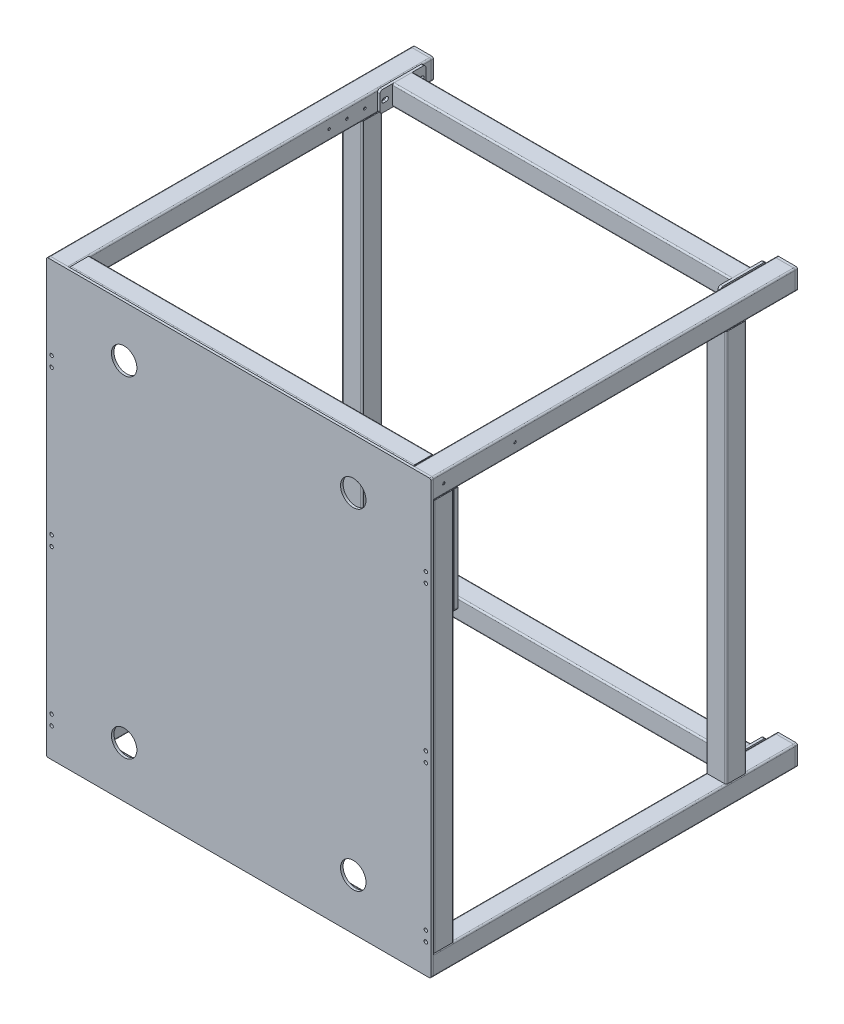
from build123d import *

# Parameters (mm, degrees)
SKETCH_1_W             = 755
SKETCH_1_H             = 850
EXTRUDE_1_DEPTH        = 5
EXTRUDE_3_DEPTH        = 710
EXTRUDE_3_2_DEPTH      = 710
EXTRUDE_3_3_DEPTH      = 710
EXTRUDE_3_4_DEPTH      = 710
FILLET_1_R             = 3
EXTRUDE_4_DEPTH        = 675
EXTRUDE_4_2_DEPTH      = 675
EXTRUDE_5_DEPTH        = 770
EXTRUDE_5_2_DEPTH      = 770
SKETCH_6_R             = 3.4
CUT_EXTRUDE_1_DEPTH    = 30
SKETCH_7_R             = 9.5
EXTRUDE_6_DEPTH        = 5
EXTRUDE_6_2_DEPTH      = 5
EXTRUDE_6_3_DEPTH      = 5
EXTRUDE_6_4_DEPTH      = 5
SKETCH_8_W             = 60
SKETCH_8_H             = 210
EXTRUDE_7_DEPTH        = 8
SKETCH_9_R             = 3.4
CUT_EXTRUDE_2_DEPTH    = 10
FILLET_2_R             = 5
EXTRUDE_8_DEPTH        = 770
EXTRUDE_8_2_DEPTH      = 770
SKETCH_11_W            = 90
SKETCH_11_H            = 40
EXTRUDE_9_DEPTH        = 5
FILLET_3_R             = 5
CUT_EXTRUDE_3_DEPTH    = 5
EXTRUDE_10_DEPTH       = 664
EXTRUDE_11_DEPTH       = 5
CUT_EXTRUDE_START      = -2
SKETCH_15_R            = 2.5
CUT_EXTRUDE_4_DEPTH    = 679
PATTERN_LINEAR_1_COUNT = 2
PATTERN_LINEAR_1_PITCH = 810
SKETCH_16_R            = 25
CUT_EXTRUDE_5_DEPTH    = 10
SKETCH_17_R            = 2.5
CUT_EXTRUDE_6_DEPTH    = 1.5


with BuildPart() as part:
    # 草图1 → 凸台-拉伸1 (new body)
    with BuildSketch(Plane.XY):
        Rectangle(SKETCH_1_W, SKETCH_1_H)
    extrude(amount=EXTRUDE_1_DEPTH)

    # 圆角1
    fillet_1_edges = [part.edges().sort_by_distance(p)[0] for p in [
        (377.5, -425, 2.5),
        (-377.5, -425, 2.5),
        (-377.5, 425, 2.5),
        (377.5, 425, 2.5),
    ]]
    fillet(fillet_1_edges, radius=FILLET_1_R)


with BuildPart() as body_2:
    # 草图3 → 凸台-拉伸3 (new body)
    with BuildSketch(Plane(origin=(0, 0, 0), x_dir=(-1, 0, 0), z_dir=(0, 0, -1))):
        with BuildLine():
            Line((374.5, 385), (340.5, 385))
            ThreePointArc((340.5, 385), (338.378679656, 385.878679656), (337.5, 388))
            Line((337.5, 388), (337.5, 422))
            ThreePointArc((337.5, 422), (338.378679656, 424.121320344), (340.5, 425))
            Line((340.5, 425), (374.5, 425))
            ThreePointArc((374.5, 425), (376.621320344, 424.121320344), (377.5, 422))
            Line((377.5, 422), (377.5, 388))
            ThreePointArc((377.5, 388), (376.621320344, 385.878679656), (374.5, 385))
        make_face()
        with BuildLine():
            Line((339.5, 388), (339.5, 422))
            ThreePointArc((339.5, 422), (339.792893219, 422.707106781), (340.5, 423))
            Line((340.5, 423), (374.5, 423))
            ThreePointArc((374.5, 423), (375.207106781, 422.707106781), (375.5, 422))
            Line((375.5, 422), (375.5, 388))
            ThreePointArc((375.5, 388), (375.207106781, 387.292893219), (374.5, 387))
            Line((374.5, 387), (340.5, 387))
            ThreePointArc((340.5, 387), (339.792893219, 387.292893219), (339.5, 388))
        make_face(mode=Mode.SUBTRACT)
    extrude(amount=EXTRUDE_3_DEPTH)


with BuildPart() as body_3:
    # 草图3 → Extrude 3 2 (new body)
    with BuildSketch(Plane(origin=(0, 0, 0), x_dir=(-1, 0, 0), z_dir=(0, 0, -1))):
        with BuildLine():
            Line((374.5, -425), (340.5, -425))
            ThreePointArc((340.5, -425), (338.378679656, -424.121320344), (337.5, -422))
            Line((337.5, -422), (337.5, -388))
            ThreePointArc((337.5, -388), (338.378679656, -385.878679656), (340.5, -385))
            Line((340.5, -385), (374.5, -385))
            ThreePointArc((374.5, -385), (376.621320344, -385.878679656), (377.5, -388))
            Line((377.5, -388), (377.5, -422))
            ThreePointArc((377.5, -422), (376.621320344, -424.121320344), (374.5, -425))
        make_face()
        with BuildLine():
            Line((339.5, -422), (339.5, -388))
            ThreePointArc((339.5, -388), (339.792893219, -387.292893219), (340.5, -387))
            Line((340.5, -387), (374.5, -387))
            ThreePointArc((374.5, -387), (375.207106781, -387.292893219), (375.5, -388))
            Line((375.5, -388), (375.5, -422))
            ThreePointArc((375.5, -422), (375.207106781, -422.707106781), (374.5, -423))
            Line((374.5, -423), (340.5, -423))
            ThreePointArc((340.5, -423), (339.792893219, -422.707106781), (339.5, -422))
        make_face(mode=Mode.SUBTRACT)
    extrude(amount=EXTRUDE_3_2_DEPTH)


with BuildPart() as body_4:
    # 草图3 → Extrude 3 3 (new body)
    with BuildSketch(Plane(origin=(0, 0, 0), x_dir=(-1, 0, 0), z_dir=(0, 0, -1))):
        with BuildLine():
            Line((-340.5, -425), (-374.5, -425))
            ThreePointArc((-374.5, -425), (-376.621320344, -424.121320344), (-377.5, -422))
            Line((-377.5, -422), (-377.5, -388))
            ThreePointArc((-377.5, -388), (-376.621320344, -385.878679656), (-374.5, -385))
            Line((-374.5, -385), (-340.5, -385))
            ThreePointArc((-340.5, -385), (-338.378679656, -385.878679656), (-337.5, -388))
            Line((-337.5, -388), (-337.5, -422))
            ThreePointArc((-337.5, -422), (-338.378679656, -424.121320344), (-340.5, -425))
        make_face()
        with BuildLine():
            Line((-375.5, -422), (-375.5, -388))
            ThreePointArc((-375.5, -388), (-375.207106781, -387.292893219), (-374.5, -387))
            Line((-374.5, -387), (-340.5, -387))
            ThreePointArc((-340.5, -387), (-339.792893219, -387.292893219), (-339.5, -388))
            Line((-339.5, -388), (-339.5, -422))
            ThreePointArc((-339.5, -422), (-339.792893219, -422.707106781), (-340.5, -423))
            Line((-340.5, -423), (-374.5, -423))
            ThreePointArc((-374.5, -423), (-375.207106781, -422.707106781), (-375.5, -422))
        make_face(mode=Mode.SUBTRACT)
    extrude(amount=EXTRUDE_3_3_DEPTH)


with BuildPart() as body_5:
    # 草图3 → Extrude 3 4 (new body)
    with BuildSketch(Plane(origin=(0, 0, 0), x_dir=(-1, 0, 0), z_dir=(0, 0, -1))):
        with BuildLine():
            Line((-340.5, 385), (-374.5, 385))
            ThreePointArc((-374.5, 385), (-376.621320344, 385.878679656), (-377.5, 388))
            Line((-377.5, 388), (-377.5, 422))
            ThreePointArc((-377.5, 422), (-376.621320344, 424.121320344), (-374.5, 425))
            Line((-374.5, 425), (-340.5, 425))
            ThreePointArc((-340.5, 425), (-338.378679656, 424.121320344), (-337.5, 422))
            Line((-337.5, 422), (-337.5, 388))
            ThreePointArc((-337.5, 388), (-338.378679656, 385.878679656), (-340.5, 385))
        make_face()
        with BuildLine():
            Line((-375.5, 388), (-375.5, 422))
            ThreePointArc((-375.5, 422), (-375.207106781, 422.707106781), (-374.5, 423))
            Line((-374.5, 423), (-340.5, 423))
            ThreePointArc((-340.5, 423), (-339.792893219, 422.707106781), (-339.5, 422))
            Line((-339.5, 422), (-339.5, 388))
            ThreePointArc((-339.5, 388), (-339.792893219, 387.292893219), (-340.5, 387))
            Line((-340.5, 387), (-374.5, 387))
            ThreePointArc((-374.5, 387), (-375.207106781, 387.292893219), (-375.5, 388))
        make_face(mode=Mode.SUBTRACT)
    extrude(amount=EXTRUDE_3_4_DEPTH)


with BuildPart() as body_6:
    # 草图4 → 凸台-拉伸4 (new body)
    with BuildSketch(Plane(origin=(-337.5, 0, 0), x_dir=(0, 0, -1), z_dir=(1, 0, 0))):
        with BuildLine():
            Line((37, 385), (3, 385))
            ThreePointArc((3, 385), (0.878679656, 385.878679656), (0, 388))
            Line((0, 388), (0, 422))
            ThreePointArc((0, 422), (0.878679656, 424.121320344), (3, 425))
            Line((3, 425), (37, 425))
            ThreePointArc((37, 425), (39.121320344, 424.121320344), (40, 422))
            Line((40, 422), (40, 388))
            ThreePointArc((40, 388), (39.121320344, 385.878679656), (37, 385))
        make_face()
        with BuildLine():
            Line((2, 388), (2, 422))
            ThreePointArc((2, 422), (2.292893219, 422.707106781), (3, 423))
            Line((3, 423), (37, 423))
            ThreePointArc((37, 423), (37.707106781, 422.707106781), (38, 422))
            Line((38, 422), (38, 388))
            ThreePointArc((38, 388), (37.707106781, 387.292893219), (37, 387))
            Line((37, 387), (3, 387))
            ThreePointArc((3, 387), (2.292893219, 387.292893219), (2, 388))
        make_face(mode=Mode.SUBTRACT)
    extrude(amount=EXTRUDE_4_DEPTH)


with BuildPart() as body_7:
    # 草图4 → Extrude 4 2 (new body)
    with BuildSketch(Plane(origin=(-337.5, 0, 0), x_dir=(0, 0, -1), z_dir=(1, 0, 0))):
        with BuildLine():
            Line((37, -425), (3, -425))
            ThreePointArc((3, -425), (0.878679656, -424.121320344), (0, -422))
            Line((0, -422), (0, -388))
            ThreePointArc((0, -388), (0.878679656, -385.878679656), (3, -385))
            Line((3, -385), (37, -385))
            ThreePointArc((37, -385), (39.121320344, -385.878679656), (40, -388))
            Line((40, -388), (40, -422))
            ThreePointArc((40, -422), (39.121320344, -424.121320344), (37, -425))
        make_face()
        with BuildLine():
            Line((2, -422), (2, -388))
            ThreePointArc((2, -388), (2.292893219, -387.292893219), (3, -387))
            Line((3, -387), (37, -387))
            ThreePointArc((37, -387), (37.707106781, -387.292893219), (38, -388))
            Line((38, -388), (38, -422))
            ThreePointArc((38, -422), (37.707106781, -422.707106781), (37, -423))
            Line((37, -423), (3, -423))
            ThreePointArc((3, -423), (2.292893219, -422.707106781), (2, -422))
        make_face(mode=Mode.SUBTRACT)
    extrude(amount=EXTRUDE_4_2_DEPTH)


with BuildPart() as body_8:
    # 草图5 → 凸台-拉伸5 (new body)
    with BuildSketch(Plane(origin=(0, -385, 0), x_dir=(1, 0, 0), z_dir=(0, 1, 0))):
        with BuildLine():
            Line((374.5, 0), (340.5, 0))
            ThreePointArc((340.5, 0), (338.378679656, 0.878679656), (337.5, 3))
            Line((337.5, 3), (337.5, 37))
            ThreePointArc((337.5, 37), (338.378679656, 39.121320344), (340.5, 40))
            Line((340.5, 40), (374.5, 40))
            ThreePointArc((374.5, 40), (376.621320344, 39.121320344), (377.5, 37))
            Line((377.5, 37), (377.5, 3))
            ThreePointArc((377.5, 3), (376.621320344, 0.878679656), (374.5, 0))
        make_face()
        with BuildLine():
            Line((339.5, 3), (339.5, 37))
            ThreePointArc((339.5, 37), (339.792893219, 37.707106781), (340.5, 38))
            Line((340.5, 38), (374.5, 38))
            ThreePointArc((374.5, 38), (375.207106781, 37.707106781), (375.5, 37))
            Line((375.5, 37), (375.5, 3))
            ThreePointArc((375.5, 3), (375.207106781, 2.292893219), (374.5, 2))
            Line((374.5, 2), (340.5, 2))
            ThreePointArc((340.5, 2), (339.792893219, 2.292893219), (339.5, 3))
        make_face(mode=Mode.SUBTRACT)
    extrude(amount=EXTRUDE_5_DEPTH)


with BuildPart() as body_9:
    # 草图5 → Extrude 5 2 (new body)
    with BuildSketch(Plane(origin=(0, -385, 0), x_dir=(1, 0, 0), z_dir=(0, 1, 0))):
        with BuildLine():
            Line((-340.5, 0), (-374.5, 0))
            ThreePointArc((-374.5, 0), (-376.621320344, 0.878679656), (-377.5, 3))
            Line((-377.5, 3), (-377.5, 37))
            ThreePointArc((-377.5, 37), (-376.621320344, 39.121320344), (-374.5, 40))
            Line((-374.5, 40), (-340.5, 40))
            ThreePointArc((-340.5, 40), (-338.378679656, 39.121320344), (-337.5, 37))
            Line((-337.5, 37), (-337.5, 3))
            ThreePointArc((-337.5, 3), (-338.378679656, 0.878679656), (-340.5, 0))
        make_face()
        with BuildLine():
            Line((-375.5, 3), (-375.5, 37))
            ThreePointArc((-375.5, 37), (-375.207106781, 37.707106781), (-374.5, 38))
            Line((-374.5, 38), (-340.5, 38))
            ThreePointArc((-340.5, 38), (-339.792893219, 37.707106781), (-339.5, 37))
            Line((-339.5, 37), (-339.5, 3))
            ThreePointArc((-339.5, 3), (-339.792893219, 2.292893219), (-340.5, 2))
            Line((-340.5, 2), (-374.5, 2))
            ThreePointArc((-374.5, 2), (-375.207106781, 2.292893219), (-375.5, 3))
        make_face(mode=Mode.SUBTRACT)
    extrude(amount=EXTRUDE_5_2_DEPTH)


with BuildPart() as cut_extrude_1_tool:
    # 草图6 → 切除-拉伸1 (new body)
    with BuildSketch(Plane.XY.offset(5)):
        with Locations(Location((-367.5, -367.5, 0), (0, 0, 180))):
            Circle(SKETCH_6_R)
        with Locations(Location((-367.5, -347.5, 0), (0, 0, 180))):
            Circle(SKETCH_6_R)
        with Locations(Location((367.5, 262.5, 0), (0, 0, 180))):
            Circle(SKETCH_6_R)
        with Locations(Location((-367.5, -62.5, 0), (0, 0, 180))):
            Circle(SKETCH_6_R)
        with Locations(Location((-367.5, -42.5, 0), (0, 0, 180))):
            Circle(SKETCH_6_R)
        with Locations(Location((-367.5, 242.5, 0), (0, 0, 180))):
            Circle(SKETCH_6_R)
        with Locations(Location((-367.5, 262.5, 0), (0, 0, 180))):
            Circle(SKETCH_6_R)
        with Locations(Location((367.5, 242.5, 0), (0, 0, 180))):
            Circle(SKETCH_6_R)
        with Locations(Location((367.5, -42.5, 0), (0, 0, 180))):
            Circle(SKETCH_6_R)
        with Locations(Location((367.5, -62.5, 0), (0, 0, 180))):
            Circle(SKETCH_6_R)
        with Locations(Location((367.5, -347.5, 0), (0, 0, 180))):
            Circle(SKETCH_6_R)
        with Locations(Location((367.5, -367.5, 0), (0, 0, 180))):
            Circle(SKETCH_6_R)
    extrude(amount=-CUT_EXTRUDE_1_DEPTH)


with BuildPart() as part_1:
    add(part.part)

    # 切除-拉伸1: cut by cut_extrude_1_tool
    add(cut_extrude_1_tool.part, mode=Mode.SUBTRACT)

    # 草图16 → 切除-拉伸5 (cut)
    with BuildSketch(Plane.XY.offset(5)):
        with Locations((-225, 325)):
            Circle(SKETCH_16_R)
        with Locations((225, 325)):
            Circle(SKETCH_16_R)
        with Locations((225, -325)):
            Circle(SKETCH_16_R)
        with Locations((-225, -325)):
            Circle(SKETCH_16_R)
    extrude(amount=-CUT_EXTRUDE_5_DEPTH, mode=Mode.SUBTRACT)


with BuildPart() as body_8_1:
    add(body_8.part)

    # 切除-拉伸1: cut by cut_extrude_1_tool
    add(cut_extrude_1_tool.part, mode=Mode.SUBTRACT)


with BuildPart() as body_9_1:
    add(body_9.part)

    # 切除-拉伸1: cut by cut_extrude_1_tool
    add(cut_extrude_1_tool.part, mode=Mode.SUBTRACT)


with BuildPart() as body_10:
    # 草图7 → 凸台-拉伸6 (new body)
    with BuildSketch(Plane(origin=(0, 0, -710), x_dir=(-1, 0, 0), z_dir=(0, 0, -1))):
        with BuildLine():
            Line((337.5, 422), (337.5, 388))
            ThreePointArc((337.5, 388), (338.378679656, 385.878679656), (340.5, 385))
            Line((340.5, 385), (374.5, 385))
            ThreePointArc((374.5, 385), (376.621320344, 385.878679656), (377.5, 388))
            Line((377.5, 388), (377.5, 422))
            ThreePointArc((377.5, 422), (376.621320344, 424.121320344), (374.5, 425))
            Line((374.5, 425), (340.5, 425))
            ThreePointArc((340.5, 425), (338.378679656, 424.121320344), (337.5, 422))
        make_face()
        with Locations((357.5, 405)):
            Circle(SKETCH_7_R, mode=Mode.SUBTRACT)
    extrude(amount=EXTRUDE_6_DEPTH)


with BuildPart() as body_11:
    # 草图7 → Extrude 6 2 (new body)
    with BuildSketch(Plane(origin=(0, 0, -710), x_dir=(-1, 0, 0), z_dir=(0, 0, -1))):
        with BuildLine():
            Line((337.5, -388), (337.5, -422))
            ThreePointArc((337.5, -422), (338.378679656, -424.121320344), (340.5, -425))
            Line((340.5, -425), (374.5, -425))
            ThreePointArc((374.5, -425), (376.621320344, -424.121320344), (377.5, -422))
            Line((377.5, -422), (377.5, -388))
            ThreePointArc((377.5, -388), (376.621320344, -385.878679656), (374.5, -385))
            Line((374.5, -385), (340.5, -385))
            ThreePointArc((340.5, -385), (338.378679656, -385.878679656), (337.5, -388))
        make_face()
        with Locations((357.5, -405)):
            Circle(SKETCH_7_R, mode=Mode.SUBTRACT)
    extrude(amount=EXTRUDE_6_2_DEPTH)


with BuildPart() as body_12:
    # 草图7 → Extrude 6 3 (new body)
    with BuildSketch(Plane(origin=(0, 0, -710), x_dir=(-1, 0, 0), z_dir=(0, 0, -1))):
        with BuildLine():
            Line((-377.432040581, -388), (-377.432040581, -422))
            ThreePointArc((-377.432040581, -422), (-376.553360924, -424.121320344), (-374.432040581, -425))
            Line((-374.432040581, -425), (-340.432040581, -425))
            ThreePointArc((-340.432040581, -425), (-338.310720237, -424.121320344), (-337.432040581, -422))
            Line((-337.432040581, -422), (-337.432040581, -388))
            ThreePointArc((-337.432040581, -388), (-338.310720237, -385.878679656), (-340.432040581, -385))
            Line((-340.432040581, -385), (-374.432040581, -385))
            ThreePointArc((-374.432040581, -385), (-376.553360924, -385.878679656), (-377.432040581, -388))
        make_face()
        with Locations((-357.432040581, -405)):
            Circle(SKETCH_7_R, mode=Mode.SUBTRACT)
    extrude(amount=EXTRUDE_6_3_DEPTH)


with BuildPart() as body_13:
    # 草图7 → Extrude 6 4 (new body)
    with BuildSketch(Plane(origin=(0, 0, -710), x_dir=(-1, 0, 0), z_dir=(0, 0, -1))):
        with BuildLine():
            Line((-377.5, 422), (-377.5, 388))
            ThreePointArc((-377.5, 388), (-376.621320344, 385.878679656), (-374.5, 385))
            Line((-374.5, 385), (-340.5, 385))
            ThreePointArc((-340.5, 385), (-338.378679656, 385.878679656), (-337.5, 388))
            Line((-337.5, 388), (-337.5, 422))
            ThreePointArc((-337.5, 422), (-338.378679656, 424.121320344), (-340.5, 425))
            Line((-340.5, 425), (-374.5, 425))
            ThreePointArc((-374.5, 425), (-376.621320344, 424.121320344), (-377.5, 422))
        make_face()
        with Locations((-357.5, 405)):
            Circle(SKETCH_7_R, mode=Mode.SUBTRACT)
    extrude(amount=EXTRUDE_6_4_DEPTH)


with BuildPart() as body_14:
    # 草图8 → 凸台-拉伸7 (new body)
    with BuildSketch(Plane(origin=(0, 0, -40), x_dir=(-1, 0, 0), z_dir=(0, 0, -1))):
        with Locations((-347.5, 280)):
            Rectangle(SKETCH_8_W, SKETCH_8_H)
    extrude(amount=EXTRUDE_7_DEPTH)


with BuildPart() as cut_extrude_2_tool:
    # 草图9 → 切除-拉伸2 (new body)
    with BuildSketch(Plane(origin=(0, 0, -48), x_dir=(-1, 0, 0), z_dir=(0, 0, -1))):
        with Locations((-366.5, 187.5)):
            Circle(SKETCH_9_R)
        with Locations((-328.5, 187.5)):
            Circle(SKETCH_9_R)
        with Locations((-366.5, 352.5)):
            Circle(SKETCH_9_R)
        with Locations((-328.5, 352.5)):
            Circle(SKETCH_9_R)
    extrude(amount=-CUT_EXTRUDE_2_DEPTH)


with BuildPart() as body_8_2:
    add(body_8_1.part)

    # 切除-拉伸2: cut by cut_extrude_2_tool
    add(cut_extrude_2_tool.part, mode=Mode.SUBTRACT)


with BuildPart() as body_14_1:
    add(body_14.part)

    # 切除-拉伸2: cut by cut_extrude_2_tool
    add(cut_extrude_2_tool.part, mode=Mode.SUBTRACT)

    # 圆角2
    fillet_2_edges = [body_14_1.edges().sort_by_distance(p)[0] for p in [
        (317.5, 385, -44),
        (317.5, 175, -44),
        (377.5, 175, -44),
    ]]
    fillet(fillet_2_edges, radius=FILLET_2_R)


with BuildPart() as body_15:
    # 草图10 → 凸台-拉伸8 (new body)
    with BuildSketch(Plane.XZ.offset(-385)):
        with BuildLine():
            Line((-340.5, -615), (-374.5, -615))
            ThreePointArc((-374.5, -615), (-376.621320344, -614.121320344), (-377.5, -612))
            Line((-377.5, -612), (-377.5, -578))
            ThreePointArc((-377.5, -578), (-376.621320344, -575.878679656), (-374.5, -575))
            Line((-374.5, -575), (-340.5, -575))
            ThreePointArc((-340.5, -575), (-338.378679656, -575.878679656), (-337.5, -578))
            Line((-337.5, -578), (-337.5, -612))
            ThreePointArc((-337.5, -612), (-338.378679656, -614.121320344), (-340.5, -615))
        make_face()
        with BuildLine():
            Line((-375.5, -612), (-375.5, -578))
            ThreePointArc((-375.5, -578), (-375.207106781, -577.292893219), (-374.5, -577))
            Line((-374.5, -577), (-340.5, -577))
            ThreePointArc((-340.5, -577), (-339.792893219, -577.292893219), (-339.5, -578))
            Line((-339.5, -578), (-339.5, -612))
            ThreePointArc((-339.5, -612), (-339.792893219, -612.707106781), (-340.5, -613))
            Line((-340.5, -613), (-374.5, -613))
            ThreePointArc((-374.5, -613), (-375.207106781, -612.707106781), (-375.5, -612))
        make_face(mode=Mode.SUBTRACT)
    extrude(amount=EXTRUDE_8_DEPTH)


with BuildPart() as body_16:
    # 草图10 → Extrude 8 2 (new body)
    with BuildSketch(Plane.XZ.offset(-385)):
        with BuildLine():
            Line((374.5, -615), (340.5, -615))
            ThreePointArc((340.5, -615), (338.378679656, -614.121320344), (337.5, -612))
            Line((337.5, -612), (337.5, -578))
            ThreePointArc((337.5, -578), (338.378679656, -575.878679656), (340.5, -575))
            Line((340.5, -575), (374.5, -575))
            ThreePointArc((374.5, -575), (376.621320344, -575.878679656), (377.5, -578))
            Line((377.5, -578), (377.5, -612))
            ThreePointArc((377.5, -612), (376.621320344, -614.121320344), (374.5, -615))
        make_face()
        with BuildLine():
            Line((339.5, -612), (339.5, -578))
            ThreePointArc((339.5, -578), (339.792893219, -577.292893219), (340.5, -577))
            Line((340.5, -577), (374.5, -577))
            ThreePointArc((374.5, -577), (375.207106781, -577.292893219), (375.5, -578))
            Line((375.5, -578), (375.5, -612))
            ThreePointArc((375.5, -612), (375.207106781, -612.707106781), (374.5, -613))
            Line((374.5, -613), (340.5, -613))
            ThreePointArc((340.5, -613), (339.792893219, -612.707106781), (339.5, -612))
        make_face(mode=Mode.SUBTRACT)
    extrude(amount=EXTRUDE_8_2_DEPTH)


with BuildPart() as body_17:
    # 草图11 → 凸台-拉伸9 (new body)
    with BuildSketch(Plane(origin=(-337.5, 0, 0), x_dir=(0, 0, -1), z_dir=(1, 0, 0))):
        with Locations((650, -405)):
            Rectangle(SKETCH_11_W, SKETCH_11_H)
    extrude(amount=EXTRUDE_9_DEPTH)

    # 圆角3
    fillet_3_edges = [body_17.edges().sort_by_distance(p)[0] for p in [
        (-335, -385, -605),
        (-335, -385, -695),
        (-335, -425, -695),
        (-335, -425, -605),
    ]]
    fillet(fillet_3_edges, radius=FILLET_3_R)

    # 草图12 → 切除-拉伸3 (cut)
    with BuildSketch(Plane(origin=(-332.5, 0, 0), x_dir=(0, 0, -1), z_dir=(1, 0, 0))):
        with BuildLine():
            Line((612.5, -401), (617.5, -401))
            ThreePointArc((617.5, -401), (621.5, -405), (617.5, -409))
            Line((617.5, -409), (612.5, -409))
            ThreePointArc((612.5, -409), (608.5, -405), (612.5, -401))
        make_face()
        with BuildLine():
            Line((687.5, -401), (682.5, -401))
            ThreePointArc((682.5, -401), (678.5, -405), (682.5, -409))
            Line((682.5, -409), (687.5, -409))
            ThreePointArc((687.5, -409), (691.5, -405), (687.5, -401))
        make_face()
    extrude(amount=-CUT_EXTRUDE_3_DEPTH, mode=Mode.SUBTRACT)


with BuildPart() as body_18:
    # 草图13 → 凸台-拉伸10 (new body)
    with BuildSketch(Plane(origin=(-332.5, 0, 0), x_dir=(0, 0, -1), z_dir=(1, 0, 0))):
        with BuildLine():
            Line((667, -425), (633, -425))
            ThreePointArc((633, -425), (630.878679656, -424.121320344), (630, -422))
            Line((630, -422), (630, -388))
            ThreePointArc((630, -388), (630.878679656, -385.878679656), (633, -385))
            Line((633, -385), (667, -385))
            ThreePointArc((667, -385), (669.121320344, -385.878679656), (670, -388))
            Line((670, -388), (670, -422))
            ThreePointArc((670, -422), (669.121320344, -424.121320344), (667, -425))
        make_face()
        with BuildLine():
            Line((632, -422), (632, -388))
            ThreePointArc((632, -388), (632.292893219, -387.292893219), (633, -387))
            Line((633, -387), (667, -387))
            ThreePointArc((667, -387), (667.707106781, -387.292893219), (668, -388))
            Line((668, -388), (668, -422))
            ThreePointArc((668, -422), (667.707106781, -422.707106781), (667, -423))
            Line((667, -423), (633, -423))
            ThreePointArc((633, -423), (632.292893219, -422.707106781), (632, -422))
        make_face(mode=Mode.SUBTRACT)
    extrude(amount=EXTRUDE_10_DEPTH)


with BuildPart() as body_19:
    # 草图14 → 凸台-拉伸11 (new body)
    with BuildSketch(Plane(origin=(331.5, 0, 0), x_dir=(0, 0, -1), z_dir=(1, 0, 0))):
        with BuildLine():
            Line((610, -425), (690, -425))
            ThreePointArc((690, -425), (693.535533906, -423.535533906), (695, -420))
            Line((695, -420), (695, -390))
            ThreePointArc((695, -390), (693.535533906, -386.464466094), (690, -385))
            Line((690, -385), (610, -385))
            ThreePointArc((610, -385), (606.464466094, -386.464466094), (605, -390))
            Line((605, -390), (605, -420))
            ThreePointArc((605, -420), (606.464466094, -423.535533906), (610, -425))
        make_face()
        with BuildLine():
            Line((687.5, -401), (682.5, -401))
            ThreePointArc((682.5, -401), (678.5, -405), (682.5, -409))
            Line((682.5, -409), (687.5, -409))
            ThreePointArc((687.5, -409), (691.5, -405), (687.5, -401))
        make_face(mode=Mode.SUBTRACT)
        with BuildLine():
            Line((612.5, -409), (617.5, -409))
            ThreePointArc((617.5, -409), (621.5, -405), (617.5, -401))
            Line((617.5, -401), (612.5, -401))
            ThreePointArc((612.5, -401), (608.5, -405), (612.5, -409))
        make_face(mode=Mode.SUBTRACT)
    extrude(amount=EXTRUDE_11_DEPTH)


with BuildPart() as cut_extrude_4_tool:
    # 草图15 → 切除-拉伸4 (new body)
    with BuildSketch(Plane(origin=(-337.5, 0, 0), x_dir=(0, 0, -1), z_dir=(1, 0, 0)).offset(CUT_EXTRUDE_START)):
        with Locations((685, -405)):
            Circle(SKETCH_15_R)
        with Locations((650, -405)):
            Circle(SKETCH_15_R)
        with Locations((615, -405)):
            Circle(SKETCH_15_R)
        with Locations((580, -405)):
            Circle(SKETCH_15_R)
        with Locations((545, -405)):
            Circle(SKETCH_15_R)
        with Locations((510, -405)):
            Circle(SKETCH_15_R)
        with Locations((510, 405)):
            Circle(SKETCH_15_R)
        with Locations((545, 405)):
            Circle(SKETCH_15_R)
        with Locations((580, 405)):
            Circle(SKETCH_15_R)
        with Locations((615, 405)):
            Circle(SKETCH_15_R)
        with Locations((650, 405)):
            Circle(SKETCH_15_R)
        with Locations((685, 405)):
            Circle(SKETCH_15_R)
    extrude(amount=CUT_EXTRUDE_4_DEPTH)


with BuildPart() as body_2_1:
    add(body_2.part)

    # 切除-拉伸4: cut by cut_extrude_4_tool
    add(cut_extrude_4_tool.part, mode=Mode.SUBTRACT)


with BuildPart() as body_3_1:
    add(body_3.part)

    # 切除-拉伸4: cut by cut_extrude_4_tool
    add(cut_extrude_4_tool.part, mode=Mode.SUBTRACT)


with BuildPart() as body_4_1:
    add(body_4.part)

    # 切除-拉伸4: cut by cut_extrude_4_tool
    add(cut_extrude_4_tool.part, mode=Mode.SUBTRACT)


with BuildPart() as body_5_1:
    add(body_5.part)

    # 切除-拉伸4: cut by cut_extrude_4_tool
    add(cut_extrude_4_tool.part, mode=Mode.SUBTRACT)

    # 草图17 → 切除-拉伸6 (cut)
    with BuildSketch(Plane(origin=(377.5, 0, 0), x_dir=(0, 0, -1), z_dir=(1, 0, 0))):
        with Locations((20, 405)):
            Circle(SKETCH_17_R)
        with Locations((160, 405)):
            Circle(SKETCH_17_R)
    extrude(amount=-CUT_EXTRUDE_6_DEPTH, mode=Mode.SUBTRACT)


with BuildPart() as body_17_1:
    add(body_17.part)

    # 切除-拉伸4: cut by cut_extrude_4_tool
    add(cut_extrude_4_tool.part, mode=Mode.SUBTRACT)


with BuildPart() as body_19_1:
    add(body_19.part)

    # 切除-拉伸4: cut by cut_extrude_4_tool
    add(cut_extrude_4_tool.part, mode=Mode.SUBTRACT)


with BuildPart() as pattern_linear_1_1:
    # 阵列(线性)1: pattern copy
    add(body_19_1.part.moved(Location(Vector(0, 1, 0) * (1 * PATTERN_LINEAR_1_PITCH))))


with BuildPart() as pattern_linear_1_2:
    # 阵列(线性)1: pattern copy
    add(body_17_1.part.moved(Location(Vector(0, 1, 0) * (1 * PATTERN_LINEAR_1_PITCH))))


with BuildPart() as pattern_linear_1_3:
    # 阵列(线性)1: pattern copy
    add(body_18.part.moved(Location(Vector(0, 1, 0) * (1 * PATTERN_LINEAR_1_PITCH))))


solid = Compound([body_6.part, body_7.part, part_1.part, body_9_1.part, body_10.part, body_11.part, body_12.part, body_13.part, body_8_2.part, body_14_1.part, body_15.part, body_16.part, body_18.part, body_2_1.part, body_3_1.part, body_4_1.part, body_5_1.part, body_17_1.part, body_19_1.part, pattern_linear_1_1.part, pattern_linear_1_2.part, pattern_linear_1_3.part])
